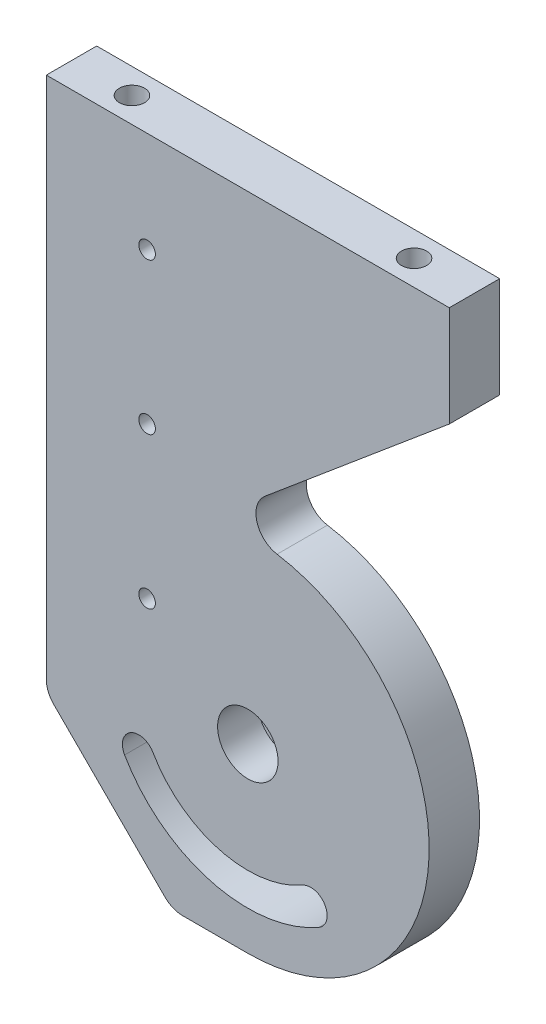
from build123d import *

# Parameters (mm, degrees)
SKETCH_1_W                = 80
SKETCH_1_H                = 170
EXTRUDE_1_DEPTH           = 5
HOLE_WIZARD_1_D           = 10
HOLE_WIZARD_1_CBORE_D     = 12
HOLE_WIZARD_1_CBORE_DEPTH = 8
CUT_EXTRUDE_2_DEPTH       = 95.472218138
CUT_EXTRUDE_4_DEPTH       = 95.472218138
FILLET_1_R                = 5
HOLE_WIZARD_M6_1_D        = 5
HOLE_WIZARD_M6_1_DEPTH    = 17
HOLE_WIZARD_M6_1_TIP      = 1.502151548
HOLE_WIZARD_M4_1_D        = 3.3


with BuildPart() as part:
    # 草图1 → 凸台-拉伸1 (new, symmetric)
    with BuildSketch(Plane.XY):
        Rectangle(SKETCH_1_W, SKETCH_1_H)
    extrude(amount=EXTRUDE_1_DEPTH, both=True)

    # 孔1 (through all)
    with Locations(Plane(origin=(0, 0, 5), x_dir=(-1, 0, 0), z_dir=(0, 0, 1))):
        with Locations((0, 10)):
            CounterBoreHole(HOLE_WIZARD_1_D / 2, HOLE_WIZARD_1_CBORE_D / 2, HOLE_WIZARD_1_CBORE_DEPTH)

    # 草图6 → 切除-拉伸2 (cut, through all)
    with BuildSketch(Plane(origin=(0, 0, -5), x_dir=(-1, 0, 0), z_dir=(0, 0, -1))):
        with BuildLine():
            ThreePointArc((-14.125, -34.465217657), (7.311638024, -37.287404593), (24.465217657, -24.125))
            ThreePointArc((24.465217657, -24.125), (23.275635095, -19.685417438), (18.836052532, -20.875))
            ThreePointArc((18.836052532, -20.875), (5.629314231, -31.008886722), (-10.875, -28.836052532))
            ThreePointArc((-10.875, -28.836052532), (-15.314582562, -30.025635095), (-14.125, -34.465217657))
        make_face()
    extrude(amount=-CUT_EXTRUDE_2_DEPTH, mode=Mode.SUBTRACT)

    # 草图11 → 切除-拉伸4 (cut, through all)
    with BuildSketch(Plane(origin=(0, 0, -5), x_dir=(-1, 0, 0), z_dir=(0, 0, -1))):
        with BuildLine():
            Line((0, -46), (15, -46))
            Line((15, -46), (40, -21))
            Line((40, -21), (40, -85))
            Line((40, -85), (-40, -85))
            Line((-40, -85), (-40, 65))
            Line((-40, 65), (7.392754444, 25.232757226))
            ThreePointArc((7.392754444, 25.232757226), (-35.807675575, -6.283769392), (0, -46))
        make_face()
    extrude(amount=-CUT_EXTRUDE_4_DEPTH, mode=Mode.SUBTRACT)

    # 圆角1
    fillet_1_edges = [part.edges().sort_by_distance(p)[0] for p in [
        (-40, -21, 0),
        (-7.392754444, 25.232757226, 0),
        (-15, -46, 0),
    ]]
    fillet(fillet_1_edges, radius=FILLET_1_R)

    # M6 螺纹孔1
    with Locations(Plane(origin=(0, 85, 0), x_dir=(1, 0, 0), z_dir=(0, 1, 0))):
        with Locations((-28, 0), (28, 0)):
            Hole(HOLE_WIZARD_M6_1_D / 2, depth=HOLE_WIZARD_M6_1_DEPTH)
            with Locations((0, 0, -(HOLE_WIZARD_M6_1_DEPTH + HOLE_WIZARD_M6_1_TIP / 2))):  # 118° drill point
                Cone(0, HOLE_WIZARD_M6_1_D / 2, HOLE_WIZARD_M6_1_TIP, mode=Mode.SUBTRACT)

    # M4 螺纹孔1 (through all)
    with Locations(Plane(origin=(0, 0, -5), x_dir=(-1, 0, 0), z_dir=(0, 0, -1))):
        with Locations((20, 35), (20, 65), (20, 5)):
            Hole(HOLE_WIZARD_M4_1_D / 2)


solid = part.part
